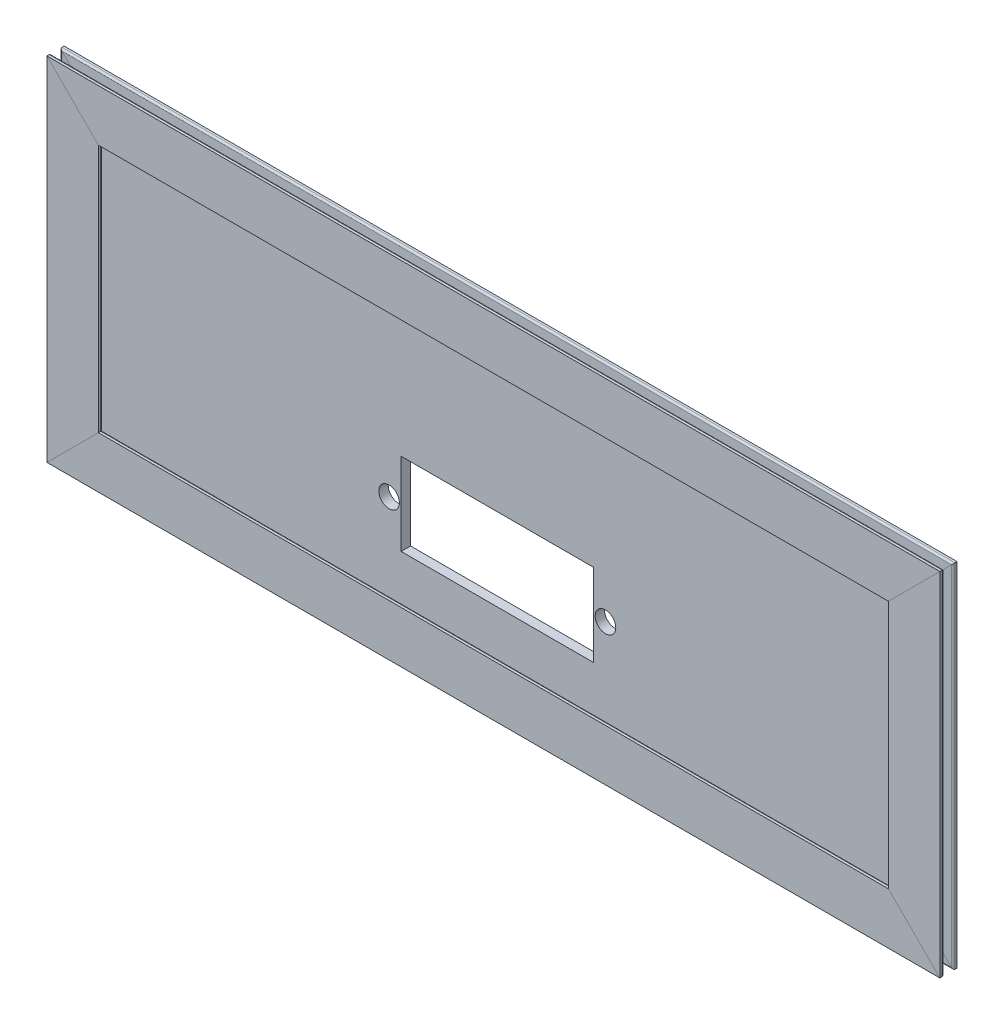
SolidWorks part; units mm, degrees
ref_plane "Front Plane" through (0, 0, 0) normal (0, 0, 1) x (1, 0, 0)
ref_plane "Top Plane" through (0, 0, 0) normal (0, 1, 0) x (1, 0, 0)
ref_plane "Right Plane" through (0, 0, 0) normal (1, 0, 0) x (0, 0, -1)
sketch "Sketch 1" plane through (0, 0, 0) normal (0, 0, 1) x (1, 0, 0)
  line L1 (-245, -87.5) -> (245, -87.5)
  line L2 (-245, -87.5) -> (-245, 87.5)
  line L3 (-245, 87.5) -> (245, 87.5)
  line L4 (245, -87.5) -> (245, 87.5)
  line L5 (-245, -87.5) -> (245, 87.5) construction
  line L6 (-245, 87.5) -> (245, -87.5) construction
  point P0 (0, 0)
  dimension "D1" = 490
  dimension "D2" = 175
other "Aluminium profile 20 X 20 X 2(1)"
ref_plane "Plane1" through (-245, 87.5, 0) normal (1, 0, 0) x (0, 1, 0)
sketch "Sketch1" plane through (-245, 87.5, 0) normal (1, 0, 0) x (0, 1, 0)
  line L0 (-3.1, -2.2) -> (3.1, -2.2)
  line L1 (3.1, -2.2) -> (3.1, 2.2)
  line L2 (3.1, 2.2) -> (-3.1, 2.2)
  line L3 (-3.1, 2.2) -> (-3.1, -2.2)
  line L4 (4.5, 2.75) -> (14, 2.75)
  line L5 (4.5, -2.75) -> (4.5, 2.75)
  line L6 (14, -2.75) -> (4.5, -2.75)
  line L7 (15, -5) -> (15, -3.75)
  line L8 (-15, -5) -> (15, -5)
  line L9 (-15, -3.75) -> (-15, -5)
  line L10 (-4.5, -2.75) -> (-14, -2.75)
  line L11 (-4.5, 2.75) -> (-4.5, -2.75)
  line L12 (-14, 2.75) -> (-4.5, 2.75)
  line L13 (-15, 5) -> (-15, 3.75)
  line L14 (15, 5) -> (-15, 5)
  line L15 (15, 3.75) -> (15, 5)
  arc A0 (15, -3.75) -> (14, -2.75) centre (14, -3.75) ccw
  arc A1 (-14, -2.75) -> (-15, -3.75) centre (-14, -3.75) ccw
  arc A2 (-15, 3.75) -> (-14, 2.75) centre (-14, 3.75) ccw
  arc A3 (14, 2.75) -> (15, 3.75) centre (14, 3.75) ccw
  point P24 (0, 0)
sketch "Sketch3" plane through (0, 0, -2.75) normal (0, 0, 1) x (1, 0, 0)
  line L1 (-231, 73.5) -> (231, 73.5)
  line L2 (-231, 73.5) -> (-231, -73.5)
  line L3 (-231, -73.5) -> (231, -73.5)
  line L4 (231, 73.5) -> (231, -73.5)
extrude "Boss-Extrude1" add sketch "Sketch3" along normal up to surface (5.5 mm away) separate body up to face at (0, -78.25, 2.75)
sketch "Sketch4" plane through (0, 0, -2.75) normal (0, 0, -1) x (-1, 0, 0)
  line L0 (230, -72.5) -> (-230, -72.5) construction
  line L1 (56, -46.5) -> (-56, -46.5)
  line L2 (56, -46.5) -> (56, 1.5)
  line L3 (56, 1.5) -> (-56, 1.5)
  line L4 (-56, -46.5) -> (-56, 1.5)
  line L5 (56, -46.5) -> (-56, 1.5) construction
  line L6 (56, 1.5) -> (-56, -46.5) construction
  line L7 (-63, -22.5) -> (63, -22.5) construction
  line L8 (0, 0) -> (0, -22.5) construction
  circle A0 centre (-63, -22.5) radius 6
  circle A1 centre (63, -22.5) radius 6
  point P0 (0, -22.5)
  point P15 (0, -22.5)
  dimension "D5" = 12
  dimension "D1" = 50
  dimension "D2" = 112
  dimension "D3" = 48
  dimension "D4" = 126
extrude "Cut-Extrude1" cut sketch "Sketch4" against normal through all
